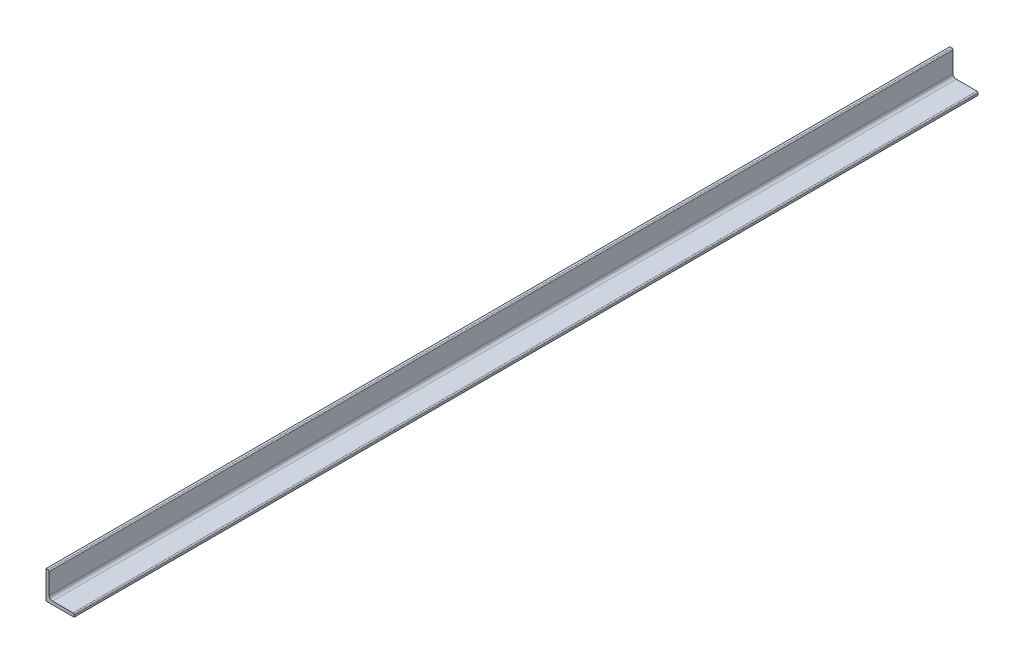
from build123d import *

# Parameters (mm, degrees)
BOSS_EXTRUDE1_DEPTH = 2250


with BuildPart() as part:
    # Sketch1 → Boss-Extrude1 (new body)
    with BuildSketch(Plane.XY):
        with BuildLine():
            Line((0, 70), (0, 0))
            Line((0, 0), (70, 0))
            Line((70, 0), (70, 5))
            ThreePointArc((70, 5), (69.121320344, 7.121320344), (67, 8))
            Line((67, 8), (16, 8))
            ThreePointArc((16, 8), (10.343145751, 10.343145751), (8, 16))
            Line((8, 16), (8, 67))
            ThreePointArc((8, 67), (7.121320344, 69.121320344), (5, 70))
            Line((5, 70), (0, 70))
        make_face()
    extrude(amount=BOSS_EXTRUDE1_DEPTH)


solid = part.part
